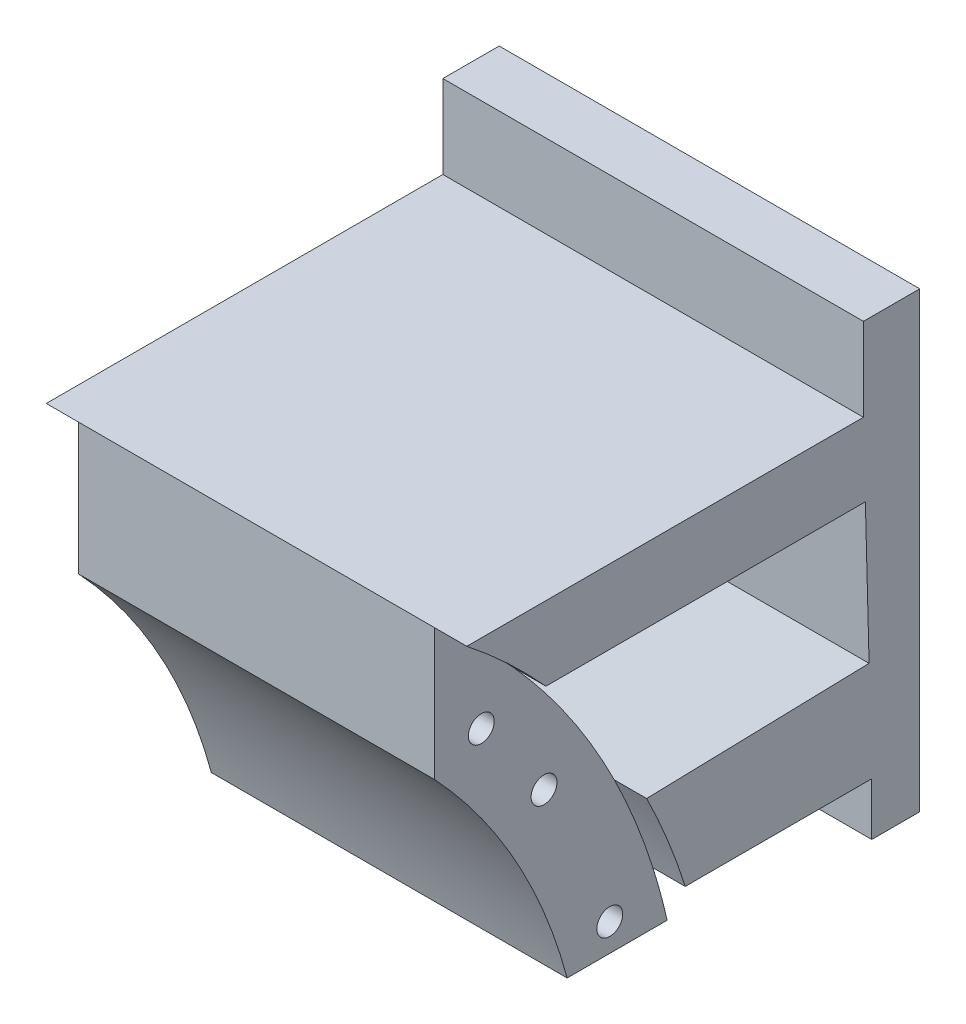
SolidWorks part; units mm, degrees
ref_plane "Front Plane" through (0, 0, 0) normal (0, 0, 1) x (1, 0, 0)
ref_plane "Top Plane" through (0, 0, 0) normal (0, 1, 0) x (1, 0, 0)
ref_plane "Right Plane" through (0, 0, 0) normal (1, 0, 0) x (0, 0, -1)
sketch "Sketch1" plane through (0, 0, 0) normal (0, 0, 1) x (1, 0, 0)
  line L4 (0, 230) -> (0, 90)
  line L5 (0, 90) -> (130, 90)
  line L6 (130, 90) -> (130, 230)
  line L7 (130, 230) -> (0, 230)
  line L8 (0, 230) -> (0, 90)
  line L9 (0, 90) -> (130, 90)
  line L10 (130, 90) -> (130, 230)
  line L11 (130, 230) -> (0, 230)
  dimension "D1" = 0
extrude "Boss-Extrude1" add sketch "Sketch1" along normal blind 10
sketch "Sketch14" plane through (0, 0, 10) normal (0, 0, 1) x (1, 0, 0)
  line L1 (130, 230) -> (0, 230)
  line L2 (130, 230) -> (130, 90)
  line L3 (130, 90) -> (0, 90)
  line L4 (0, 230) -> (0, 90)
extrude "Boss-Extrude2" add sketch "Sketch14" along normal blind 130
sketch "Sketch15" plane through (130, 0, 0) normal (1, 0, 0) x (0, 0, -1)
  line L0 (-140, 90) -> (-140, 163.653)
  line L2 (-140, 90) -> (-98.9821, 90)
  line L4 (-68.0823, 90) -> (-14.84, 90)
  line L5 (-140, 90) -> (0, 90) construction
  line L6 (-14.84, 90) -> (-14.84, 106.2643)
  line L7 (-14.84, 106.2643) -> (-72.4863, 106.2643)
  line L8 (-140, 230) -> (-140, 204.3101)
  line L9 (-140, 90) -> (-140, 230) construction
  line L10 (-140, 204.3101) -> (-17.4081, 204.3101)
  line L11 (-17.4081, 204.3101) -> (-17.4081, 230)
  line L12 (-140, 230) -> (0, 230) construction
  line L13 (-17.4081, 230) -> (-140, 230)
  line L14 (-16.8078, 181.3923) -> (-15.6601, 137.5742)
  line L15 (-16.8078, 181.3923) -> (-115.5538, 181.3923)
  line L16 (-15.6601, 137.5742) -> (-84.4186, 135.7732)
  arc A0 (-98.9821, 90) -> (-140, 163.653) centre (-266.344, 45.043) ccw
  arc A1 (-68.0823, 90) -> (-72.4863, 106.2643) centre (-266.344, 45.043) ccw
  arc A2 (-353.991, -104.4533) -> (-178.697, 194.5392) centre (-266.344, 45.043) ccw construction
  arc A3 (-84.4186, 135.7732) -> (-115.5538, 181.3923) centre (-266.344, 45.043) ccw
extrude "Cut-Extrude2" cut sketch "Sketch15" against normal through all both and the other way through all
sketch "Sketch17" plane through (130, 0, 0) normal (1, 0, 0) x (0, 0, -1)
  line L9 (-140, 204.3101) -> (-140, 163.653)
  line L10 (-98.9821, 90) -> (-68.0823, 90)
  line L11 (-72.4863, 106.2643) -> (-14.84, 106.2643)
  line L12 (-14.84, 106.2643) -> (-14.84, 90)
  line L13 (-14.84, 90) -> (0, 90)
  line L14 (0, 90) -> (0, 230)
  line L15 (0, 230) -> (-17.4081, 230)
  line L16 (-17.4081, 230) -> (-17.4081, 204.3101)
  line L17 (-17.4081, 204.3101) -> (-140, 204.3101)
  line L18 (-140, 204.3101) -> (-140, 163.653)
  line L19 (-98.9821, 90) -> (-68.0823, 90)
  arc A0 (-140, 204.3101) -> (-72.4863, 106.2643) centre (-266.344, 45.043) cw
  arc A2 (-98.9821, 90) -> (-140, 163.653) centre (-266.344, 45.043) ccw
  arc A3 (-68.0823, 90) -> (-72.4863, 106.2643) centre (-266.344, 45.043) ccw
  arc A4 (-98.9821, 90) -> (-140, 163.653) centre (-266.344, 45.043) ccw
  arc A5 (-68.0823, 90) -> (-72.4863, 106.2643) centre (-266.344, 45.043) ccw
  dimension "D1" = 0
extrude "Cut-Extrude4" cut sketch "Sketch17" against normal blind 10 and the other way through all
sketch "Sketch18" plane through (0, 0, 0) normal (-1, 0, 0) x (0, 0, 1)
  line L0 (98.9821, 90) -> (68.0823, 90)
  line L1 (140, 163.653) -> (140, 204.3101)
  arc A0 (140, 204.3101) -> (68.0823, 90) centre (266.344, 45.043) ccw
  arc A1 (140, 163.653) -> (98.9821, 90) centre (266.344, 45.043) ccw
extrude "Cut-Extrude5" cut sketch "Sketch18" against normal blind 10
sketch "Sketch19" plane through (10, 0, 0) normal (-1, 0, 0) x (0, 0, 1)
  arc A0 (128.2062, 172.9997) -> (84.7122, 94.6905) centre (266.344, 45.043) ccw construction
  arc A1 (140, 163.653) -> (98.9821, 90) centre (266.344, 45.043) ccw construction
  circle A3 centre (85.8078, 98.5376) radius 4
  circle A4 centre (106.1325, 143.9736) radius 4
  circle A5 centre (125.5193, 170.0365) radius 4
  dimension "D1" = 15
  dimension "D2" = 8
extrude "Cut-Extrude6" cut sketch "Sketch19" against normal through all both and the other way through all
